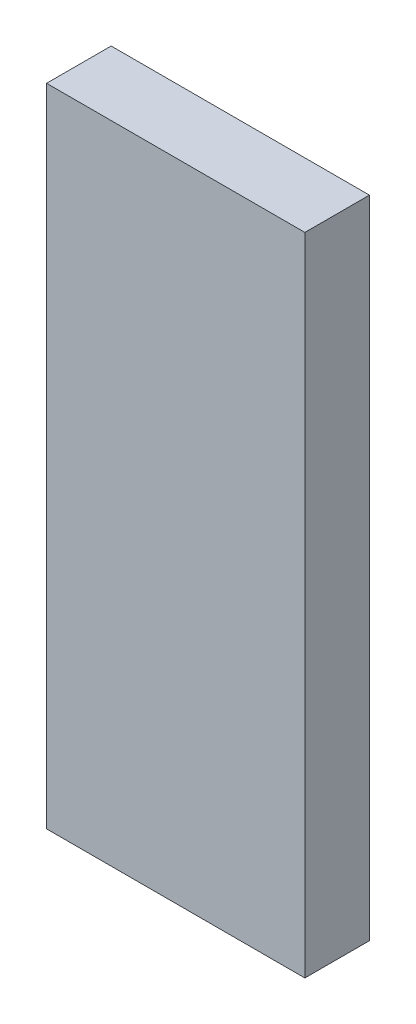
from build123d import *

# Parameters (mm, degrees)
SKETCH1_W           = 120
SKETCH1_H           = 300
BOSS_EXTRUDE1_DEPTH = 30


with BuildPart() as part:
    # Sketch1 → Boss-Extrude1 (new body)
    with BuildSketch(Plane.XY):
        with Locations((60, 150)):
            Rectangle(SKETCH1_W, SKETCH1_H)
    extrude(amount=BOSS_EXTRUDE1_DEPTH)


solid = part.part
